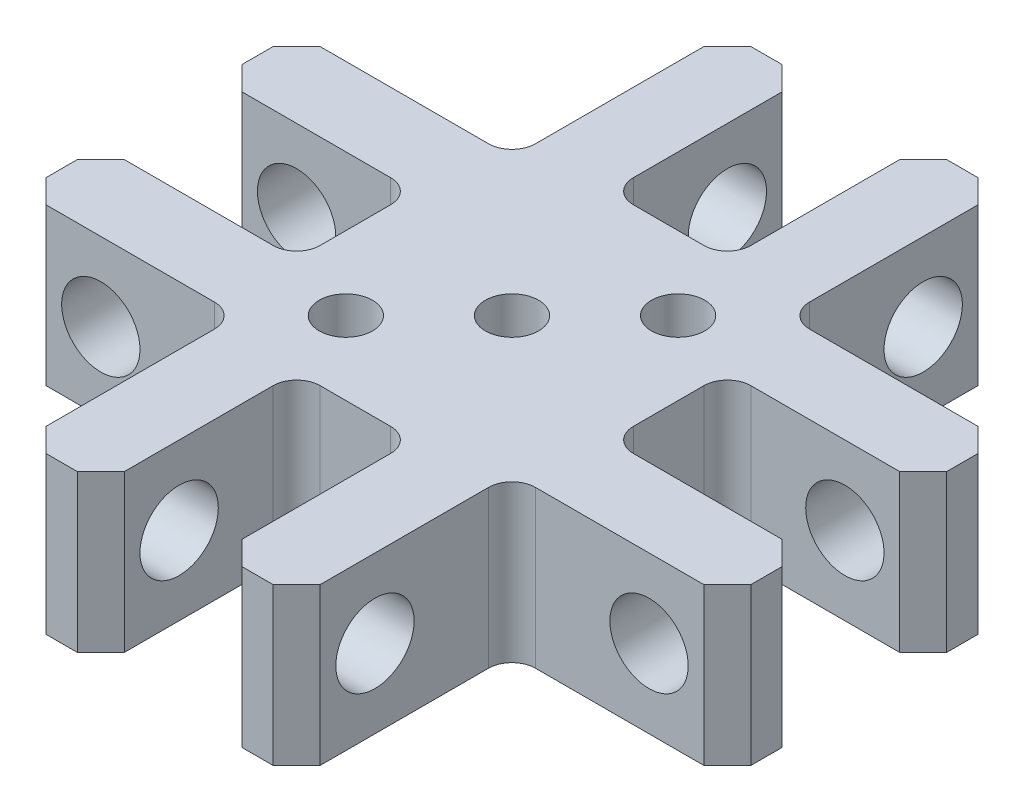
from build123d import *

# Parameters (mm, degrees)
SKETCH1_W                = 90
SKETCH1_H                = 90
BOSS_EXTRUDE1_DEPTH      = 20
CHAMFER1_SIZE            = 3
M8_TAPPED_HOLE1_D        = 6.8
M8_TAPPED_HOLE1_DEPTH    = 19.75
M8_TAPPED_HOLE1_TIP      = 2.042926105
SKETCH4_W                = 15
SKETCH4_H                = 25
CUT_EXTRUDE1_DEPTH       = 42
FILLET1_R                = 3
CHAMFER2_SIZE            = 3
CIRPATTERN2_COUNT        = 4
FILLET1_OF_CIRPATTERN2_R = 3
CHAMFER3_SIZE            = 3
SKETCH5_W                = 27.5
SKETCH5_H                = 27.5
CUT_EXTRUDE2_DEPTH       = 42
CIRPATTERN3_COUNT        = 4
CHAMFER4_SIZE            = 3
FILLET2_R                = 3
SKETCH6_R                = 5
CUT_EXTRUDE3_DEPTH       = 42
CIRPATTERN4_COUNT        = 4
M8_TAPPED_HOLE2_D        = 6.8
M8_TAPPED_HOLE2_DEPTH    = 19.75
M8_TAPPED_HOLE2_TIP      = 2.042926105


with BuildPart() as part:
    # Sketch1 → Boss-Extrude1 (new body)
    with BuildSketch(Plane(origin=(0, 0, 0), x_dir=(1, 0, 0), z_dir=(0, 1, 0))):
        Rectangle(SKETCH1_W, SKETCH1_H)
    extrude(amount=BOSS_EXTRUDE1_DEPTH)

    # Chamfer1
    chamfer1_edges = [part.edges().sort_by_distance(p)[0] for p in [
        (-45, 10, -45),
        (45, 10, -45),
        (45, 10, 45),
        (-45, 10, 45),
    ]]
    chamfer(chamfer1_edges, length=CHAMFER1_SIZE)

    # M8 Tapped Hole1
    with Locations(Plane(origin=(0, 20, 0), x_dir=(1, 0, 0), z_dir=(0, 1, 0))):
        with Locations((0, 0)):
            Hole(M8_TAPPED_HOLE1_D / 2, depth=M8_TAPPED_HOLE1_DEPTH)
            with Locations((0, 0, -(M8_TAPPED_HOLE1_DEPTH + M8_TAPPED_HOLE1_TIP / 2))):  # 118° drill point
                Cone(0, M8_TAPPED_HOLE1_D / 2, M8_TAPPED_HOLE1_TIP, mode=Mode.SUBTRACT)

    # Sketch4 → Cut-Extrude1 (cut)
    with BuildSketch(Plane(origin=(0, 20, 0), x_dir=(1, 0, 0), z_dir=(0, 1, 0))):
        with Locations((0, 32.5)):
            Rectangle(SKETCH4_W, SKETCH4_H)
    cut_extrude1 = extrude(amount=-CUT_EXTRUDE1_DEPTH, mode=Mode.SUBTRACT)

    # Fillet1
    fillet1_edges = [part.edges().sort_by_distance(p)[0] for p in [
        (7.5, 10, -20),
        (-7.5, 10, -20),
    ]]
    fillet(fillet1_edges, radius=FILLET1_R)

    # Chamfer2
    chamfer2_edges = [part.edges().sort_by_distance(p)[0] for p in [
        (7.5, 10, -45),
        (-7.5, 10, -45),
    ]]
    chamfer(chamfer2_edges, length=CHAMFER2_SIZE)

    # CirPattern2: Cut-Extrude1 ×4 about axis
    cirpattern2_axis = Axis((0, 0, 0), (0, 1, 0))
    for i in range(1, CIRPATTERN2_COUNT):
        add(cut_extrude1.rotate(cirpattern2_axis, i * 360 / CIRPATTERN2_COUNT), mode=Mode.SUBTRACT)

    # Fillet1 of CirPattern2
    fillet1_of_cirpattern2_edges = [part.edges().sort_by_distance(p)[0] for p in [
        (-20, 10, -7.5),
        (-20, 10, 7.5),
        (-7.5, 10, 20),
        (7.5, 10, 20),
        (20, 10, 7.5),
        (20, 10, -7.5),
    ]]
    fillet(fillet1_of_cirpattern2_edges, radius=FILLET1_OF_CIRPATTERN2_R)

    # Chamfer3
    chamfer3_edges = [part.edges().sort_by_distance(p)[0] for p in [
        (-45, 10, -7.5),
        (-45, 10, 7.5),
        (-7.5, 10, 45),
        (7.5, 10, 45),
        (45, 10, 7.5),
        (45, 10, -7.5),
    ]]
    chamfer(chamfer3_edges, length=CHAMFER3_SIZE)

    # Sketch5 → Cut-Extrude2 (cut)
    with BuildSketch(Plane(origin=(0, 20, 0), x_dir=(1, 0, 0), z_dir=(0, 1, 0))):
        with Locations((-31.25, 31.25)):
            Rectangle(SKETCH5_W, SKETCH5_H)
    cut_extrude2 = extrude(amount=-CUT_EXTRUDE2_DEPTH, mode=Mode.SUBTRACT)

    # CirPattern3: Cut-Extrude2 ×4 about axis
    cirpattern3_axis = Axis((0, 0, 0), (0, 1, 0))
    for i in range(1, CIRPATTERN3_COUNT):
        add(cut_extrude2.rotate(cirpattern3_axis, i * 360 / CIRPATTERN3_COUNT), mode=Mode.SUBTRACT)

    # Chamfer4
    chamfer4_edges = [part.edges().sort_by_distance(p)[0] for p in [
        (-17.5, 10, -45),
        (-45, 10, -17.5),
        (-45, 10, 17.5),
        (-17.5, 10, 45),
        (17.5, 10, 45),
        (45, 10, 17.5),
        (45, 10, -17.5),
        (17.5, 10, -45),
    ]]
    chamfer(chamfer4_edges, length=CHAMFER4_SIZE)

    # Fillet2
    fillet2_edges = [part.edges().sort_by_distance(p)[0] for p in [
        (-17.5, 10, -17.5),
        (-17.5, 10, 17.5),
        (17.5, 10, 17.5),
        (17.5, 10, -17.5),
    ]]
    fillet(fillet2_edges, radius=FILLET2_R)

    # Sketch6 → Cut-Extrude3 (cut)
    with BuildSketch(Plane.ZY.offset(17.5)):
        with Locations((-35, 10)):
            Circle(SKETCH6_R)
    cut_extrude3 = extrude(amount=-CUT_EXTRUDE3_DEPTH, mode=Mode.SUBTRACT)

    # CirPattern4: Cut-Extrude3 ×4 about axis
    cirpattern4_axis = Axis((0, 20, 0), (0, 1, 0))
    for i in range(1, CIRPATTERN4_COUNT):
        add(cut_extrude3.rotate(cirpattern4_axis, i * 360 / CIRPATTERN4_COUNT), mode=Mode.SUBTRACT)

    # M8 Tapped Hole2
    with Locations(Plane(origin=(0, 20, 0), x_dir=(1, 0, 0), z_dir=(0, 1, 0))):
        with Locations((-10.606601718, -10.606601718), (10.606601718, 10.606601718)):
            Hole(M8_TAPPED_HOLE2_D / 2, depth=M8_TAPPED_HOLE2_DEPTH)
            with Locations((0, 0, -(M8_TAPPED_HOLE2_DEPTH + M8_TAPPED_HOLE2_TIP / 2))):  # 118° drill point
                Cone(0, M8_TAPPED_HOLE2_D / 2, M8_TAPPED_HOLE2_TIP, mode=Mode.SUBTRACT)


solid = part.part
